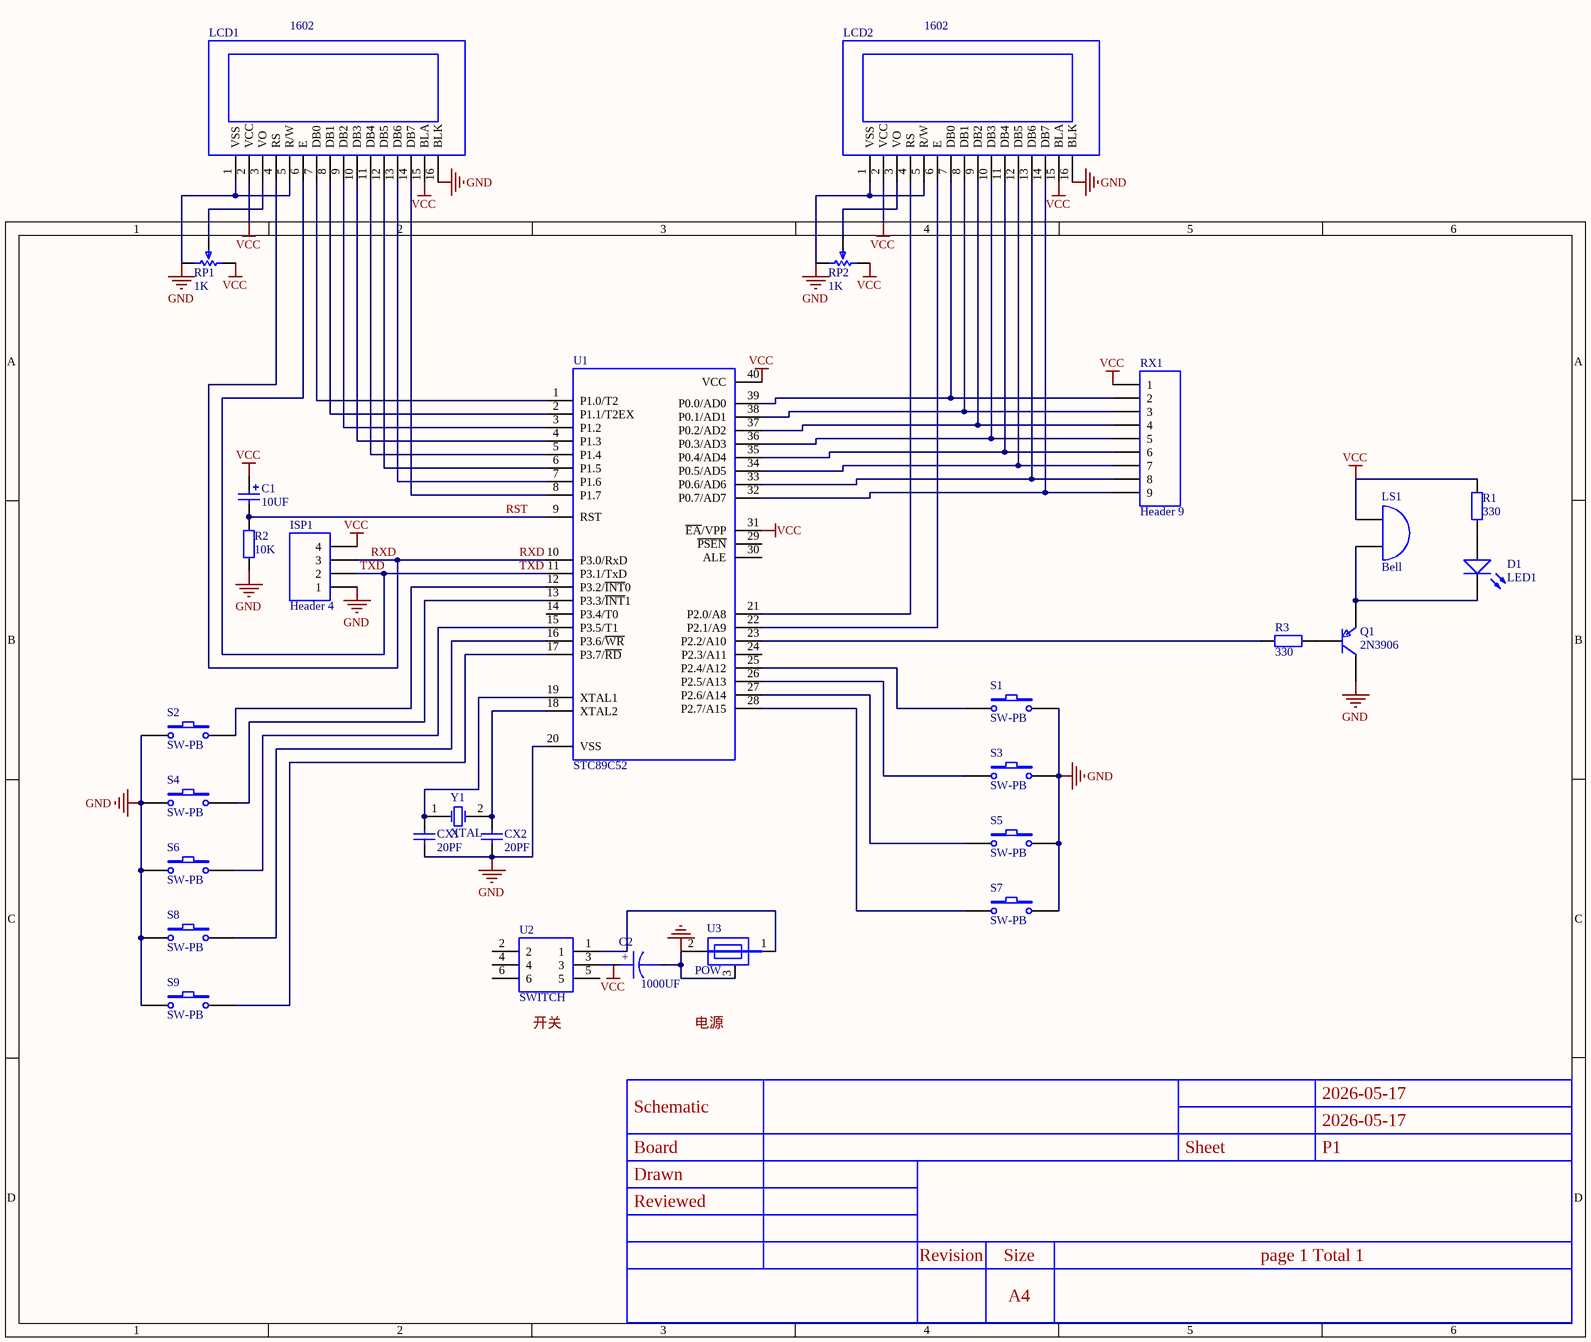
[diagram p0: MISC61252-3.schdoc]
# Altium project MISC61252-2.PrjPcb
1 sheet, 29 parts. Net scope: global (net labels, ports and power ports of the same name join across sheets).
Board file: MISC61252.pcbdoc

## Sheet MISC61252-3.schdoc
size 297 x 209 mm; Version: V1.0; @Project Name: MISC61252; @Update Date: 2026-05-17; @Create Date: 2026-05-17; @Board Name: MISC61252; @Create Time: 17:12:08; @Page Count: 1; @Page No: 1; @Schematic Name: MISC61252; @Update Time: 17:12:08; Size: A4

### Parts
C1  value 10UF  [CAP-TH_BD5.0-P2.00-D0.8-FD-10UF50VC110GL]  (hidden comment: Cap Pol2)
C2  1000UF  [CAP-TH_BD5.0-P2.00-D0.8-FD-10UF50VC110GL]
CX1  value 20PF  [CAP-TH_L5.0-W2.5-P5.00-D1.0]  (hidden comment: Cap)
CX2  value 20PF  [CAP-TH_L5.0-W2.5-P5.00-D1.0]  (hidden comment: Cap)
D1  LED1  [LED_TH-3mm]
ISP1  Header 4  [HDR-TH_4P-P2.54-V-F]
LCD1  1602  [LCD1602]
LCD2  1602  [LCD1602]
LS1  Bell  [BUZ-TH_BD12.0-P6.00-D0.9-RD]
Q1  2N3906  [TO-92-3_L4.6-W3.6-P1.27-L_1]
R1  value 330  [Res_1/8W]  (hidden comment: Res2)
R2  value 10K  [Res_1/8W]  (hidden comment: Res2)
R3  value 330  [Res_1/8W]  (hidden comment: Res2)
RP1  value 1K  [RES-ADJ-SMD_RM065-V1]  (hidden comment: RPot)
RP2  value 1K  [RES-ADJ-SMD_RM065-V1]  (hidden comment: RPot)
RX1  Header 9  [HDR-TH_9P-P2.54-V-F-1]
S1  SW-PB  [SW-TH_4P-L6.0-W6.0-P4.50-LS6.5]
S2  SW-PB  [SW-TH_4P-L6.0-W6.0-P4.50-LS6.5]
S3  SW-PB  [SW-TH_4P-L6.0-W6.0-P4.50-LS6.5]
S4  SW-PB  [SW-TH_4P-L6.0-W6.0-P4.50-LS6.5]
S5  SW-PB  [SW-TH_4P-L6.0-W6.0-P4.50-LS6.5]
S6  SW-PB  [SW-TH_4P-L6.0-W6.0-P4.50-LS6.5]
S7  SW-PB  [SW-TH_4P-L6.0-W6.0-P4.50-LS6.5]
S8  SW-PB  [SW-TH_4P-L6.0-W6.0-P4.50-LS6.5]
S9  SW-PB  [SW-TH_4P-L6.0-W6.0-P4.50-LS6.5]
U1  STC89C52  [DIP-40_L52.0-W13.7-P2.54-LS15.2-BL]
U2  SWITCH  [SW-TH_6P-L5.8-W5.8-P2.00-LS4.5-BL]
U3  POW  [DC-IN-TH_DC005]
Y1  XTAL  [HC-49S_L11.5-W5.0-P4.88]

### Nets
GND: C2.2 CX1.1 CX2.1 ISP1.1 LCD1.1(VSS) LCD1.5(R/W) LCD1.16(BLK) LCD2.1(VSS) LCD2.5(R/W) LCD2.16(BLK) Q1.3(C) R2.1 RP1.2(BOT) RP2.2(BOT) S1.2 S2.2 S3.2 S4.2 S5.2 S6.2 S7.2 S8.2 S9.2 U1.20(VSS) U3.2 U3.3
VCC: C1.1 C2.1 ISP1.4 LCD1.2(VCC) LCD1.15(BLA) LCD2.2(VCC) LCD2.15(BLA) LS1.1(A) R1.2 RP1.1(TOP) RP2.1(TOP) RX1.1 U1.31(~{EA}/VPP) U1.40(VCC) U2.3
RST: C1.2 R2.2 U1.9(RST)
RXD: ISP1.3 LCD1.4(RS) U1.10(P3.0/RxD)
TXD: ISP1.2 LCD1.6(E) U1.11(P3.1/TxD)
NetCX1_2: CX1.2 U1.19(XTAL1) Y1.1(OSC1)
NetCX2_2: CX2.2 U1.18(XTAL2) Y1.2(OSC2)
NetD1_1: D1.1(A) R1.1
NetD1_2: D1.2(K) LS1.2(B) Q1.1(E)
NetLCD1_3: LCD1.3(VO) RP1.3(TAP)
NetLCD1_7: LCD1.7(DB0) U1.1(P1.0/T2)
NetLCD1_8: LCD1.8(DB1) U1.2(P1.1/T2EX)
NetLCD1_9: LCD1.9(DB2) U1.3(P1.2)
NetLCD1_10: LCD1.10(DB3) U1.4(P1.3)
NetLCD1_11: LCD1.11(DB4) U1.5(P1.4)
NetLCD1_12: LCD1.12(DB5) U1.6(P1.5)
NetLCD1_13: LCD1.13(DB6) U1.7(P1.6)
NetLCD1_14: LCD1.14(DB7) U1.8(P1.7)
NetLCD2_3: LCD2.3(VO) RP2.3(TAP)
NetLCD2_4: LCD2.4(RS) U1.21(P2.0/A8)
NetLCD2_6: LCD2.6(E) U1.22(P2.1/A9)
NetLCD2_7: LCD2.7(DB0) RX1.2 U1.39(P0.0/AD0)
NetLCD2_8: LCD2.8(DB1) RX1.3 U1.38(P0.1/AD1)
NetLCD2_9: LCD2.9(DB2) RX1.4 U1.37(P0.2/AD2)
NetLCD2_10: LCD2.10(DB3) RX1.5 U1.36(P0.3/AD3)
NetLCD2_11: LCD2.11(DB4) RX1.6 U1.35(P0.4/AD4)
NetLCD2_12: LCD2.12(DB5) RX1.7 U1.34(P0.5/AD5)
NetLCD2_13: LCD2.13(DB6) RX1.8 U1.33(P0.6/AD6)
NetLCD2_14: LCD2.14(DB7) RX1.9 U1.32(P0.7/AD7)
NetQ1_2: Q1.2(B) R3.2
NetR3_1: R3.1 U1.23(P2.2/A10)
NetS1_1: S1.1 U1.25(P2.4/A12)
NetS2_1: S2.1 U1.12(P3.2/~{INT}0)
NetS3_1: S3.1 U1.26(P2.5/A13)
NetS4_1: S4.1 U1.13(P3.3/~{INT}1)
NetS5_1: S5.1 U1.27(P2.6/A14)
NetS6_1: S6.1 U1.15(P3.5/T1)
NetS7_1: S7.1 U1.28(P2.7/A15)
NetS8_1: S8.1 U1.16(P3.6/~{WR})
NetS9_1: S9.1 U1.17(P3.7/~{RD})
NetU2_1: U2.1 U3.1

Not connected (* = marked no-connect by the designer): U1 14(P3.4/T0) 24(P2.3/A11) 29(~{PSEN}) 30(ALE); U2 2 4 5 6

### Notes on the sheet
- Labels drawn without touching a wire or pin: 开关, 电源
- 2026-05-17
- Schematic
- Board
- Sheet
- P1
- Drawn
- Reviewed
- Revision
- Size
- A4
- page 1 Total 1

### Library data of the parts
C1 = Cap Pol2: Polarized Capacitor (Axial); Origin Footprint: POLAR0.8; AddInBom: yes; Symbol: Cap Pol2; Device: Cap Pol2; Published: 8-Jun-2000; LatestRevisionDate: 17-Jul-2002; LatestRevisionNote: Re-released for DXP Platform.; PackageReference: POLAR0.8; PackageDescription: Polarized Capacitor; 2 Leads; DesignItemID: Cap Pol2; LibraryName: Miscellaneous Devices; Publisher: Altium Limited
C2 = 10uF: Origin Footprint: C10; AddInBom: yes; Symbol: 10uF; Device: 10uF; DesignItemID: 10uF; LibraryName: *
CX1 CX2 = Cap: Capacitor; Origin Footprint: RAD-0.3; AddInBom: yes; Symbol: Cap; Device: Cap; Published: 8-Jun-2000; LatestRevisionDate: 17-Jul-2002; LatestRevisionNote: Re-released for DXP Platform.; PackageReference: RAD-0.3; PackageDescription: Radial Cap, Thru-Hole; 2 Leads; 0.3 in Pin Spacing; DesignItemID: Cap; LibraryName: Miscellaneous Devices; FootprintName: CAP-TH_L5.0-W2.5-P5.00-D1.0; Publisher: Altium Limited
D1 = LED1: Typical RED GaAs LED; Origin Footprint: LED-1; AddInBom: yes; Symbol: LED1; Device: LED1; Published: 8-Jun-2000; LatestRevisionDate: 08-Jul-2005; LatestRevisionNote: Mech Layer 1 removed.; PackageReference: LED-1; PackageDescription: LED; 2 Leads; DesignItemID: LED1; LibraryName: Miscellaneous Devices; Publisher: Altium Limited
ISP1 = Header 4: Header, 4-Pin; Origin Footprint: HDR1X4; AddInBom: yes; Symbol: Header 4; Device: Header 4; LatestRevisionDate: 17-Jul-2002; LatestRevisionNote: Re-released for DXP Platform.; DesignItemID: Header 4; LibraryName: Miscellaneous Connectors; Publisher: Altium Limited
LCD1 LCD2 = 1602: AddInBom: yes; Symbol: 1602; Device: 1602; DesignItemID: 1602; LibraryName: Schlib1
LS1 = Bell: Electrical Bell; Origin Footprint: PIN2; AddInBom: yes; Symbol: Bell; Device: Bell; Published: 24-Mar-1999; LatestRevisionDate: 17-Jul-2002; LatestRevisionNote: Re-released for DXP Platform.; PackageReference: PIN2; DesignItemID: Bell; LibraryName: Miscellaneous Devices; Publisher: Altium Limited
Q1 = 2N3906: PNP General Purpose Amplifier; Origin Footprint: TO-92A; AddInBom: yes; Symbol: 2N3906; Device: 2N3906; Published: 8-Jun-2000; LatestRevisionDate: 15-Jan-2003; LatestRevisionNote: PCB Footprint 'BCY-W3/D4.7' replaced; DatasheetVersion: 1997; PackageVersion: Sep-1998; PackageReference: TO-92A; PackageDescription: TO, Flat Index; 3 In-Line, Axial Leads; Body Dia. 4.5mm; Leads 0.51 x 0.48 mm (max); ComponentLink1Description: Manufacturer Link; ComponentLink2Description: Datasheet; DesignItemID: 2N3906; LibraryName: Miscellaneous Devices; Publisher: Altium Limited
R1 R2 = Res2: Resistor; Origin Footprint: AXIAL-0.4; AddInBom: yes; Symbol: Res2; Device: Res2; Published: 8-Jun-2000; LatestRevisionDate: 17-Jul-2002; LatestRevisionNote: Re-released for DXP Platform.; PackageReference: AXIAL-0.4; PackageDescription: Axial Device, Thru-Hole; 2 Leads; 0.4 in Pin Spacing; DesignItemID: Res2; LibraryName: Miscellaneous Devices; Publisher: Altium Limited
R3 = Res2_1: Resistor; Origin Footprint: AXIAL-0.4; AddInBom: yes; Symbol: Res2; Device: Res2_1; Published: 8-Jun-2000; LatestRevisionDate: 17-Jul-2002; LatestRevisionNote: Re-released for DXP Platform.; PackageReference: AXIAL-0.4; PackageDescription: Axial Device, Thru-Hole; 2 Leads; 0.4 in Pin Spacing; DesignItemID: Res2; LibraryName: Miscellaneous Devices; Publisher: Altium Limited
RP1 = RPot_1: Potentiometer; Sim Note: Enter the Resistance value and the set point into parameter fields.; Set Position: 0.5; Origin Footprint: VR5; AddInBom: yes; Symbol: RPot; Device: RPot_1; Published: 8-Jun-2000; LatestRevisionDate: 17-Jul-2002; LatestRevisionNote: Re-released for DXP Platform.; PackageReference: VR5; PackageDescription: Variable Resistor, Thru-Hole; 3 Leads; DesignItemID: RPot; LibraryName: Miscellaneous Devices; Publisher: Altium Limited
RP2 = RPot: Potentiometer; Sim Note: Enter the Resistance value and the set point into parameter fields.; Set Position: 0.5; Origin Footprint: VR5; AddInBom: yes; Symbol: RPot; Device: RPot; Published: 8-Jun-2000; LatestRevisionDate: 17-Jul-2002; LatestRevisionNote: Re-released for DXP Platform.; PackageReference: VR5; PackageDescription: Variable Resistor, Thru-Hole; 3 Leads; DesignItemID: RPot; LibraryName: Miscellaneous Devices; Publisher: Altium Limited
RX1 = Header 9: Header, 9-Pin; Origin Footprint: HDR1X9; AddInBom: yes; Symbol: Header 9; Device: Header 9; LatestRevisionDate: 17-Jul-2002; LatestRevisionNote: Re-released for DXP Platform.; DesignItemID: Header 9; LibraryName: Miscellaneous Connectors; Publisher: Altium Limited
S1 S3 S5 S7 = SW-PB: Switch; Origin Footprint: SPST-2; AddInBom: yes; Symbol: SW-PB; Device: SW-PB; Published: 24-Mar-1999; LatestRevisionDate: 17-Jul-2002; LatestRevisionNote: Re-released for DXP Platform.; PackageReference: SPST-2; PackageDescription: Switch; 2 Leads; DesignItemID: SW-PB; LibraryName: Miscellaneous Devices; Publisher: Altium Limited
S2 S4 S6 S8 S9 = SW-PB_1: Switch; Origin Footprint: SPST-2; AddInBom: yes; Symbol: SW-PB; Device: SW-PB_1; Published: 24-Mar-1999; LatestRevisionDate: 17-Jul-2002; LatestRevisionNote: Re-released for DXP Platform.; PackageReference: SPST-2; PackageDescription: Switch; 2 Leads; DesignItemID: SW-PB; LibraryName: Miscellaneous Devices; Publisher: Altium Limited
U1 = AT89C51: AddInBom: yes; Symbol: AT89C51; Device: AT89C51; DesignItemID: AT89C51; LibraryName: Schlib1
U2 = SWITCH: Origin Footprint: KG1; AddInBom: yes; Symbol: SWITCH; Device: SWITCH; DesignItemID: SWITCH; LibraryName: *
U3 = POW: Origin Footprint: DCM; AddInBom: yes; Symbol: POW; Device: POW; DesignItemID: POW; LibraryName: *
Y1 = XTAL: Crystal Oscillator; Origin Footprint: R38; AddInBom: yes; Symbol: XTAL; Device: XTAL; Published: 8-Jun-2000; LatestRevisionDate: 17-Jul-2002; LatestRevisionNote: Re-released for DXP Platform.; PackageReference: R38; PackageDescription: Crystal, Thru-Hole; 2 Leads; Body 3.1 x 8.2 mm (Dia.xH); DesignItemID: XTAL; LibraryName: Miscellaneous Devices; Publisher: Altium Limited